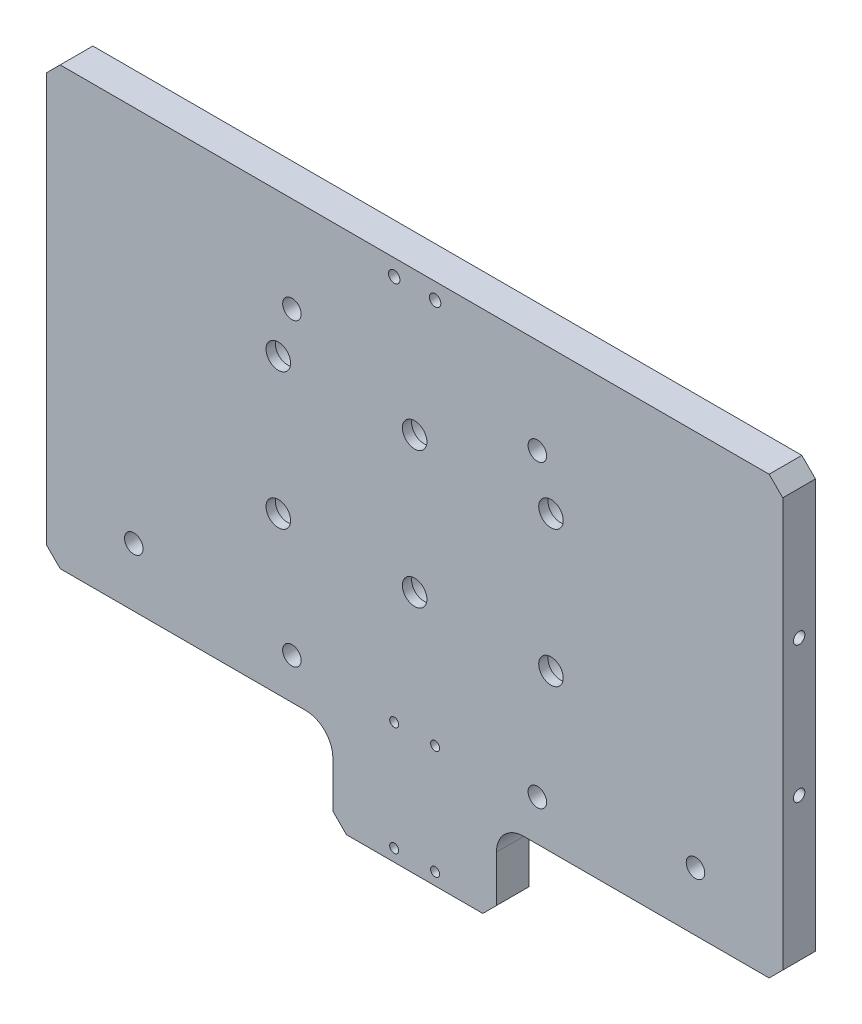
from build123d import *

# Parameters (mm, degrees)
SKETCH_1_W                   = 270
SKETCH_1_H                   = 192
EXTRUDE_1_DEPTH              = 6
SKETCH_2_W                   = 105
SKETCH_2_H                   = 32
CUT_EXTRUDE_1_DEPTH          = 12
HOLE_WIZARD_M8_1_D           = 6.8
HOLE_WIZARD_M8_1_DEPTH       = 19.75
HOLE_WIZARD_M8_1_TIP         = 2.042926105
HOLE_WIZARD_M4_1_D           = 3.3
CHAMFER_1_SIZE               = 5
FILLET_1_R                   = 10
HOLE_WIZARD_M8_2_D           = 6.8
HOLE_WIZARD_M8_3_D           = 9
HOLE_WIZARD_M8_3_DEPTH       = 24.5
HOLE_WIZARD_M8_3_CBORE_D     = 15
HOLE_WIZARD_M8_3_CBORE_DEPTH = 8.6
HOLE_WIZARD_M8_3_TIP         = 2.703872786
HOLE_WIZARD_M5_2_D           = 4.2
HOLE_WIZARD_M5_3_AT_2_COUNT  = 2
HOLE_WIZARD_M5_3_AT_2_PITCH  = 50


with BuildPart() as part:
    # 草图1 → 凸台-拉伸1 (new, symmetric)
    with BuildSketch(Plane.XY):
        Rectangle(SKETCH_1_W, SKETCH_1_H)
    extrude(amount=EXTRUDE_1_DEPTH, both=True)

    # 草图2 → 切除-拉伸1 (cut)
    with BuildSketch(Plane.XY.offset(6)):
        with Locations((-82.5, -80)):
            Rectangle(SKETCH_2_W, SKETCH_2_H)
        with Locations((82.5, -80)):
            Rectangle(SKETCH_2_W, SKETCH_2_H)
    extrude(amount=-CUT_EXTRUDE_1_DEPTH, mode=Mode.SUBTRACT)

    # M8 螺纹孔1
    with Locations(Plane.XY.offset(6)):
        with Locations((-45, 61), (45, 61)):
            Hole(HOLE_WIZARD_M8_1_D / 2, depth=HOLE_WIZARD_M8_1_DEPTH)
            with Locations((0, 0, -(HOLE_WIZARD_M8_1_DEPTH + HOLE_WIZARD_M8_1_TIP / 2))):  # 118° drill point
                Cone(0, HOLE_WIZARD_M8_1_D / 2, HOLE_WIZARD_M8_1_TIP, mode=Mode.SUBTRACT)

    # M4 螺纹孔1 (through all)
    with Locations(Plane.XY.offset(6)):
        with Locations((-7.5, -91.5), (7.5, -91.5), (-7.5, -51.5), (7.5, -51.5)):
            Hole(HOLE_WIZARD_M4_1_D / 2)

    # 倒角1
    chamfer_1_edges = [part.edges().sort_by_distance(p)[0] for p in [
        (-135, -64, 0),
        (-30, -96, 0),
        (30, -96, 0),
        (135, -64, 0),
        (-135, 96, 0),
        (135, 96, 0),
    ]]
    chamfer(chamfer_1_edges, length=CHAMFER_1_SIZE)

    # 圆角1
    fillet_1_edges = [part.edges().sort_by_distance(p)[0] for p in [
        (-30, -64, 0),
        (30, -64, 0),
    ]]
    fillet(fillet_1_edges, radius=FILLET_1_R)

    # Hole Wizard M8 _2 (through all)
    with Locations(Plane(origin=(0, 0, -6), x_dir=(-1, 0, 0), z_dir=(0, 0, -1))):
        with Locations((-45, -49), (45, -49), (-103, -42.5), (103, -42.5)):
            Hole(HOLE_WIZARD_M8_2_D / 2)

    # M8 六角凹头螺钉的柱形沉头孔3
    with Locations(Plane(origin=(0, 0, -6), x_dir=(-1, 0, 0), z_dir=(0, 0, -1))):
        with Locations((-50, 43.5), (-50, -6.5), (0, 43.5), (0, -6.5), (50, 43.5), (50, -6.5)):
            CounterBoreHole(HOLE_WIZARD_M8_3_D / 2, HOLE_WIZARD_M8_3_CBORE_D / 2, HOLE_WIZARD_M8_3_CBORE_DEPTH, depth=HOLE_WIZARD_M8_3_DEPTH)
            with Locations((0, 0, -(HOLE_WIZARD_M8_3_DEPTH + HOLE_WIZARD_M8_3_TIP / 2))):  # 118° drill point
                Cone(0, HOLE_WIZARD_M8_3_D / 2, HOLE_WIZARD_M8_3_TIP, mode=Mode.SUBTRACT)

    # M5 螺纹孔2 (through all)
    with Locations(Plane(origin=(0, 0, -6), x_dir=(-1, 0, 0), z_dir=(0, 0, -1))):
        with Locations((-7.5, 90), (7.5, 90)):
            Hole(HOLE_WIZARD_M5_2_D / 2)

    # 草图23 → M5 螺纹孔3 (revolve, cut)
    with BuildSketch(Plane(origin=(-135, -6.5, 0), x_dir=(0, 0, 1), z_dir=(0, 1, 0))):
        Polygon((0, 0), (0, 13.6618073), (2.1, 12.4), (2.1, 0), align=None)
    hole_wizard_m5_3 = revolve(axis=Axis((-141.35, -6.5, 0), (1, 0, 0)), mode=Mode.SUBTRACT)

    # M5 螺纹孔3 at 2: M5 螺纹孔3 ×2
    with Locations(*[(0, i * HOLE_WIZARD_M5_3_AT_2_PITCH, 0) for i in range(1, HOLE_WIZARD_M5_3_AT_2_COUNT)]):
        add(hole_wizard_m5_3, mode=Mode.SUBTRACT)

    # 镜向1: M5 螺纹孔3 across plane
    add(hole_wizard_m5_3.mirror(Plane(origin=(0, 0, 0), x_dir=(0, 0, 1), z_dir=(1, 0, 0))), mode=Mode.SUBTRACT)

    # 镜向1 copy 1 sketch → 镜向1 copy 1 (revolve, cut)
    with BuildSketch(Plane(origin=(135, 43.5, 0), x_dir=(0, 0, 1), z_dir=(0, 1, 0))):
        Polygon((0, 0), (0, -13.6618073), (2.1, -12.4), (2.1, 0), align=None)
    revolve(axis=Axis((141.35, 43.5, 0), (1, 0, 0)), mode=Mode.SUBTRACT)


solid = part.part
